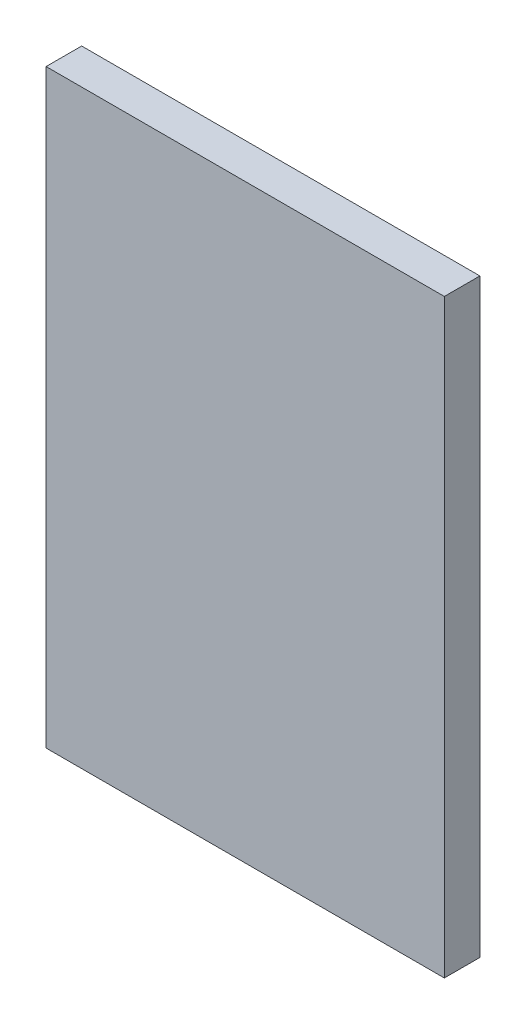
from build123d import *

# Parameters (mm, degrees)
SKETCH1_W           = 280
SKETCH1_H           = 415
BOSS_EXTRUDE1_DEPTH = 25


with BuildPart() as part:
    # Sketch1 → Boss-Extrude1 (new body)
    with BuildSketch(Plane.XY):
        Rectangle(SKETCH1_W, SKETCH1_H)
    extrude(amount=BOSS_EXTRUDE1_DEPTH)


solid = part.part
